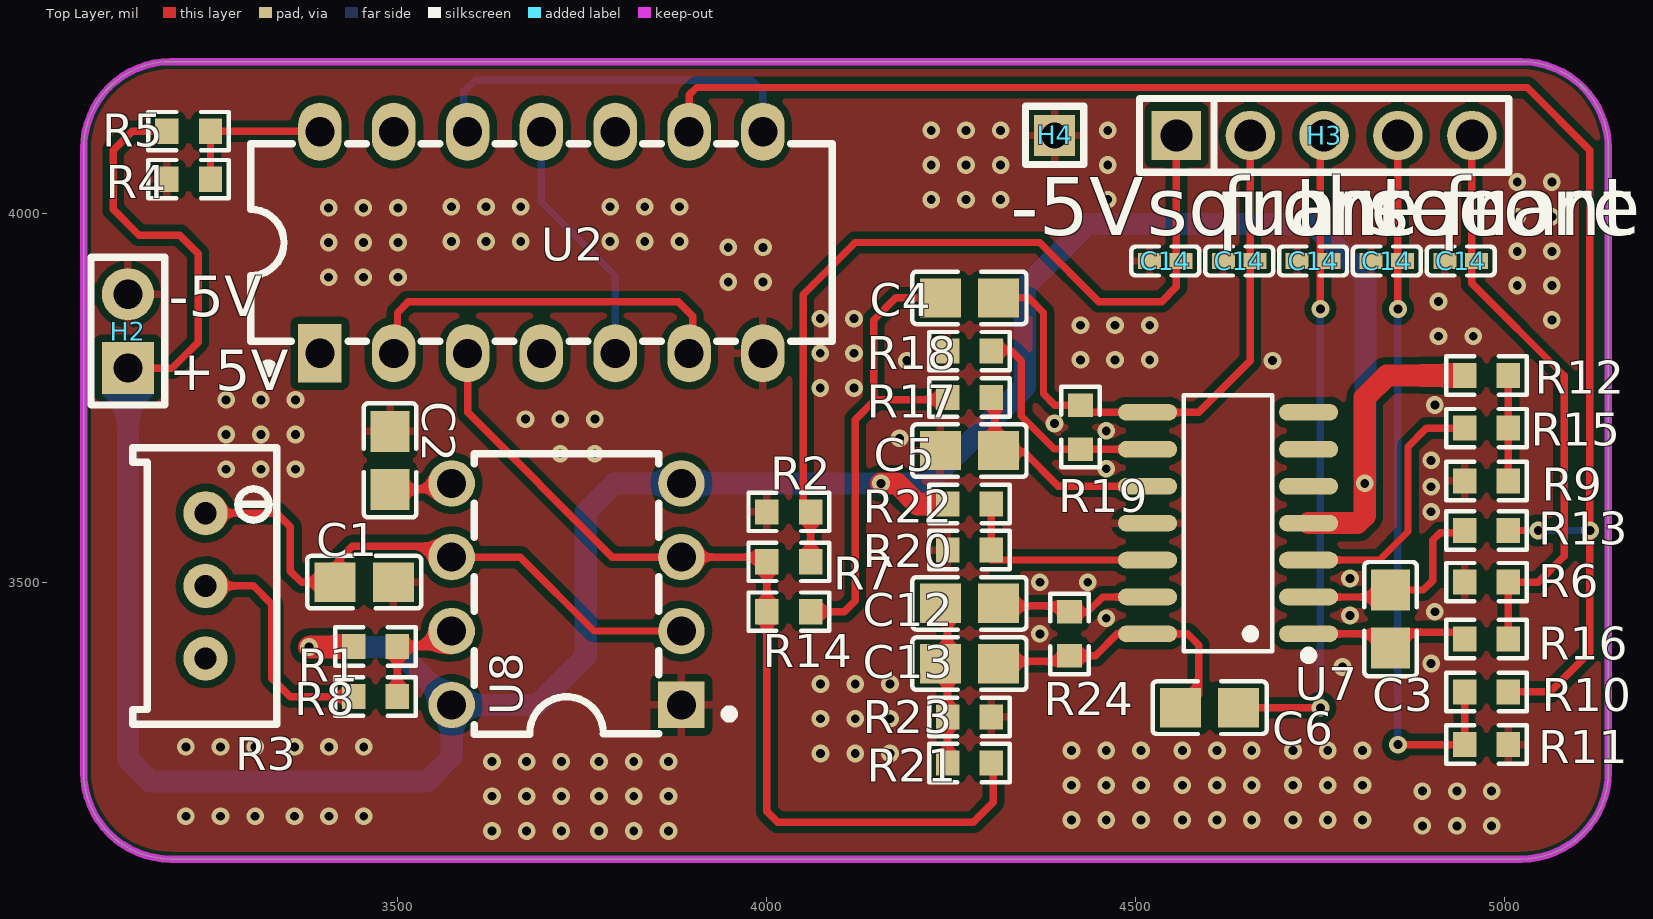
[diagram p0: Top Layer view]
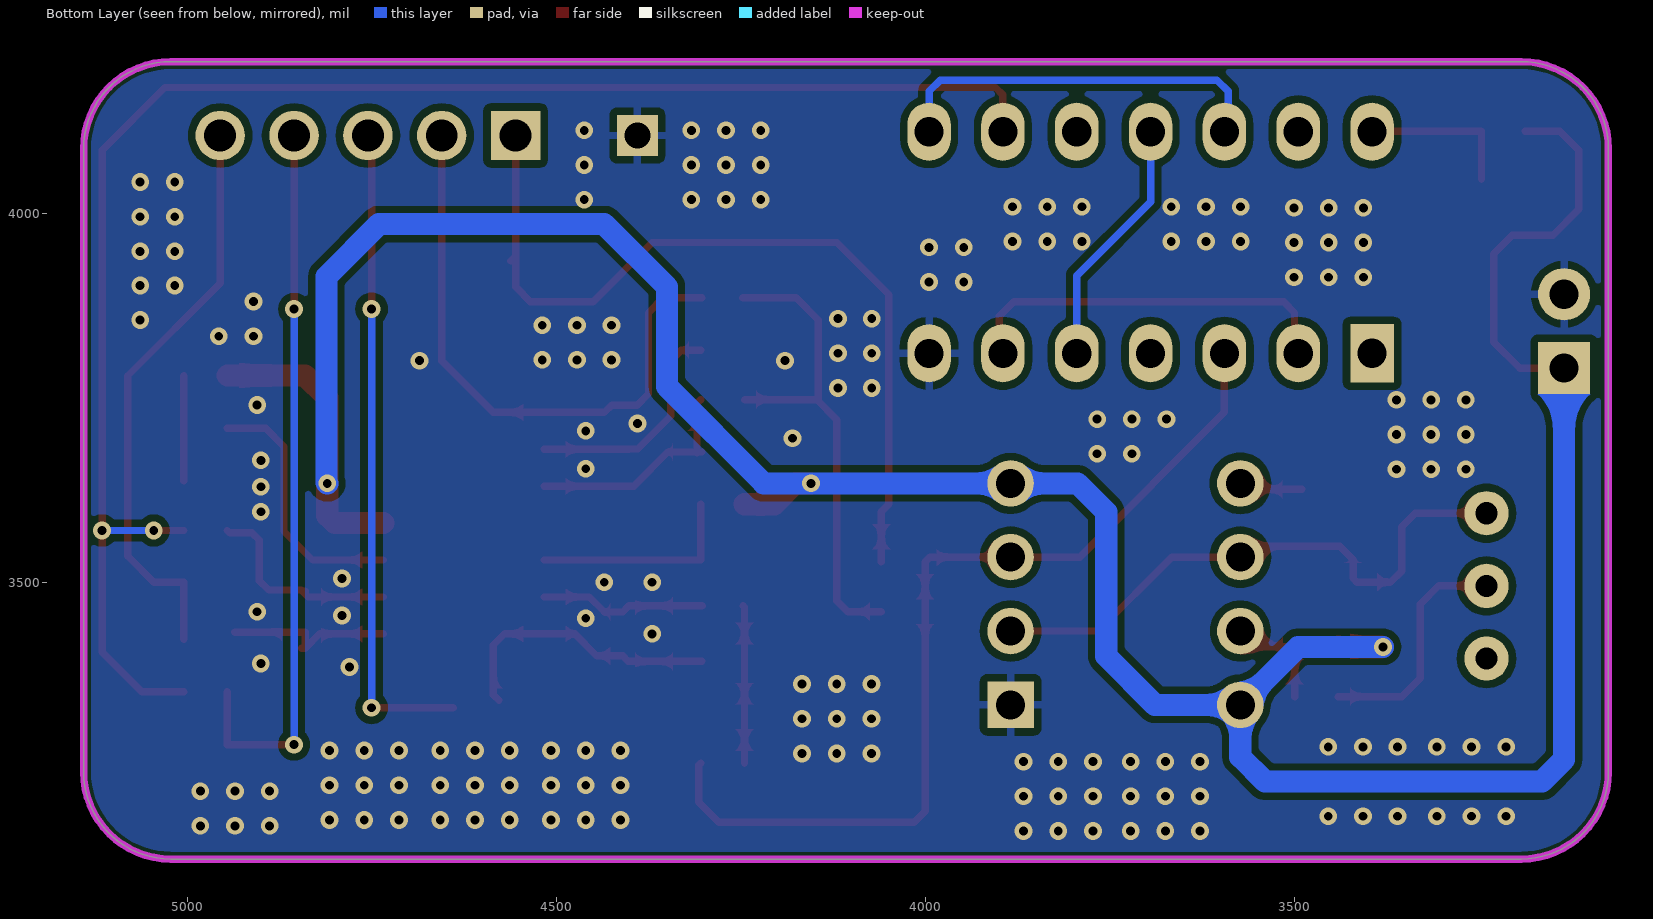
[diagram p1: Bottom Layer view, seen from below]
# Altium PCB MISC49933.pcbdoc
Units mil, origin at the board's own origin, x right, y up, seen from the top; angles counter-clockwise.
Board outline 2065 x 1080 mil, 2 copper layers (Top Layer, Bottom Layer), stack 62.206 mil thick; 43 components, 28 nets, 119 pads, 175 vias.

## Layer stack, top to bottom
Top Solder Mask Layer: solder mask 0.394, Dk 3.3
Top Layer: signal copper 1.379
Dielectric1: surface 59.449, FR4, Dk 4.5
Bottom Layer: signal copper 1.378
Bottom Solder Mask Layer: solder mask 0.394, Dk 3.3

## Board outline
3193.11,4205 ccw(c3193.11,4086.89) 3075,4086.89 3075,3243.11 ccw(c3193.11,3243.11) 3193.11,3125 5021.89,3125 ccw(c5021.89,3243.11) 5140,3243.11 5140,4086.89 ccw(c5021.89,4086.89) 5021.89,4205

## Design rules (kind name [scope] priority, off if disabled: settings)
BoardOutlineClearance copperThickness2oz_1 [All] p2 off: genericclearance=7.99 ignorepadtopadclearanceinfootprint=FALSE except(0: Arc-SplitContinuation Track-SplitContinuation SMDPad-SplitContinuation THPad-SplitContinuation Via-SplitContinuation Fill-SplitContinuation Region-SplitContinuation Poly-SplitContinuation Text-SplitContinuation Hole-SplitContinuation; 5.98: Arc-CutoutEdge Track-CutoutEdge SMDPad-CutoutEdge THPad-CutoutEdge Via-CutoutEdge Text-CutoutEdge; 6.9: Hole-OutlineEdge Hole-CutoutEdge; 10: Poly-OutlineEdge Poly-CutoutEdge; 11.81: Arc-OutlineEdge Track-OutlineEdge SMDPad-OutlineEdge THPad-OutlineEdge Via-OutlineEdge Fill-OutlineEdge Region-OutlineEdge Text-OutlineEdge Fill-CutoutEdge Region-CutoutEdge)
BoardOutlineClearance Plane_innerPlane_1 [All] p4 off: genericclearance=4.02 ignorepadtopadclearanceinfootprint=FALSE except(0: Arc-SplitContinuation Track-SplitContinuation SMDPad-SplitContinuation THPad-SplitContinuation Via-SplitContinuation Fill-SplitContinuation Region-SplitContinuation Poly-SplitContinuation Text-SplitContinuation Hole-SplitContinuation; 5.98: Arc-CutoutEdge Track-CutoutEdge SMDPad-CutoutEdge THPad-CutoutEdge Via-CutoutEdge Text-CutoutEdge; 6.9: Hole-OutlineEdge Hole-CutoutEdge; 10: Poly-OutlineEdge Poly-CutoutEdge; 11.81: Arc-OutlineEdge Track-OutlineEdge SMDPad-OutlineEdge THPad-OutlineEdge Via-OutlineEdge Fill-OutlineEdge Region-OutlineEdge Text-OutlineEdge Fill-CutoutEdge Region-CutoutEdge)
BoardOutlineClearance Copper_copperRegion_1 [All] p6 off: genericclearance=4.02 ignorepadtopadclearanceinfootprint=FALSE except(0: Arc-SplitContinuation Track-SplitContinuation SMDPad-SplitContinuation THPad-SplitContinuation Via-SplitContinuation Fill-SplitContinuation Region-SplitContinuation Poly-SplitContinuation Text-SplitContinuation Hole-SplitContinuation; 5.98: Arc-CutoutEdge Track-CutoutEdge SMDPad-CutoutEdge THPad-CutoutEdge Via-CutoutEdge Text-CutoutEdge; 6.9: Hole-OutlineEdge Hole-CutoutEdge; 10: Poly-OutlineEdge Poly-CutoutEdge; 11.81: Arc-OutlineEdge Track-OutlineEdge SMDPad-OutlineEdge THPad-OutlineEdge Via-OutlineEdge Fill-OutlineEdge Region-OutlineEdge Text-OutlineEdge Fill-CutoutEdge Region-CutoutEdge)
BoardOutlineClearance copperThickness1oz_1 [All] p8: genericclearance=4.02 ignorepadtopadclearanceinfootprint=FALSE except(0: Arc-SplitContinuation Track-SplitContinuation SMDPad-SplitContinuation THPad-SplitContinuation Via-SplitContinuation Fill-SplitContinuation Region-SplitContinuation Poly-SplitContinuation Text-SplitContinuation Hole-SplitContinuation; 5.98: Arc-CutoutEdge Track-CutoutEdge SMDPad-CutoutEdge THPad-CutoutEdge Via-CutoutEdge Text-CutoutEdge; 6.9: Hole-OutlineEdge Hole-CutoutEdge; 10: Poly-OutlineEdge Poly-CutoutEdge; 11.81: Arc-OutlineEdge Track-OutlineEdge SMDPad-OutlineEdge THPad-OutlineEdge Via-OutlineEdge Fill-OutlineEdge Region-OutlineEdge Text-OutlineEdge Fill-CutoutEdge Region-CutoutEdge)
Clearance copperThickness2oz [All] p1 off: gap=7.99 ignorepadtopadclearanceinfootprint=FALSE except(5.98: SMDPad-Track SMDPad-SMDPad THPad-Track SMDPad-THPad THPad-THPad Track-Via SMDPad-Via THPad-Via Via-Via Fill-SMDPad Region-SMDPad Fill-THPad Region-THPad Fill-Via Region-Via Fill-Fill Fill-Region Region-Region Arc-Track Arc-SMDPad Arc-THPad Arc-Via Fill-Arc Region-Arc Arc-Arc Text-Track SMDPad-Text Text-THPad Text-Via Fill-Text Region-Text Arc-Text Text-Text; 6.9: Hole-Track Hole-SMDPad Hole-THPad Hole-Via Fill-Hole Region-Hole Hole-Arc Hole-Text; 10: Poly-Track Poly-SMDPad Poly-THPad Poly-Via Poly-Fill Poly-Region Poly-Poly Poly-Arc Poly-Text Poly-Hole; 11.81: Fill-Track Region-Track)
Clearance Plane_innerPlane [All] p3 off: gap=4.02 ignorepadtopadclearanceinfootprint=FALSE except(5.98: SMDPad-Track SMDPad-SMDPad THPad-Track SMDPad-THPad THPad-THPad Track-Via SMDPad-Via THPad-Via Via-Via Fill-SMDPad Region-SMDPad Fill-THPad Region-THPad Fill-Via Region-Via Fill-Fill Fill-Region Region-Region Arc-Track Arc-SMDPad Arc-THPad Arc-Via Fill-Arc Region-Arc Arc-Arc Text-Track SMDPad-Text Text-THPad Text-Via Fill-Text Region-Text Arc-Text Text-Text; 6.9: Hole-Track Hole-SMDPad Hole-THPad Hole-Via Fill-Hole Region-Hole Hole-Arc Hole-Text; 10: Poly-Track Poly-SMDPad Poly-THPad Poly-Via Poly-Fill Poly-Region Poly-Poly Poly-Arc Poly-Text Poly-Hole; 11.81: Fill-Track Region-Track)
Clearance Copper_copperRegion [All] p5 off: gap=4.02 ignorepadtopadclearanceinfootprint=FALSE except(5.98: SMDPad-Track SMDPad-SMDPad THPad-Track SMDPad-THPad THPad-THPad Track-Via SMDPad-Via THPad-Via Via-Via Fill-SMDPad Region-SMDPad Fill-THPad Region-THPad Fill-Via Region-Via Fill-Fill Fill-Region Region-Region Arc-Track Arc-SMDPad Arc-THPad Arc-Via Fill-Arc Region-Arc Arc-Arc Text-Track SMDPad-Text Text-THPad Text-Via Fill-Text Region-Text Arc-Text Text-Text; 6.9: Hole-Track Hole-SMDPad Hole-THPad Hole-Via Fill-Hole Region-Hole Hole-Arc Hole-Text; 10: Poly-Track Poly-SMDPad Poly-THPad Poly-Via Poly-Fill Poly-Region Poly-Poly Poly-Arc Poly-Text Poly-Hole; 11.81: Fill-Track Region-Track)
Clearance copperThickness1oz [All] p7: gap=4.02 ignorepadtopadclearanceinfootprint=FALSE except(5.98: SMDPad-Track SMDPad-SMDPad THPad-Track SMDPad-THPad THPad-THPad Track-Via SMDPad-Via THPad-Via Via-Via Fill-SMDPad Region-SMDPad Fill-THPad Region-THPad Fill-Via Region-Via Fill-Fill Fill-Region Region-Region Arc-Track Arc-SMDPad Arc-THPad Arc-Via Fill-Arc Region-Arc Arc-Arc Text-Track SMDPad-Text Text-THPad Text-Via Fill-Text Region-Text Arc-Text Text-Text; 6.9: Hole-Track Hole-SMDPad Hole-THPad Hole-Via Fill-Hole Region-Hole Hole-Arc Hole-Text; 10: Poly-Track Poly-SMDPad Poly-THPad Poly-Via Poly-Fill Poly-Region Poly-Poly Poly-Arc Poly-Text Poly-Hole; 11.81: Fill-Track Region-Track)
DiffPairsRouting differentialPair [All] p1: maxlimit=6 minlimit=6 mostfreqgap=6 toplayer_minwidth=5 toplayer_prefwidth=10 toplayer_maxwidth=100 toplayer_mingap=6 toplayer_prefgap=6 toplayer_maxgap=6 bottomlayer_minwidth=5 bottomlayer_prefwidth=10 bottomlayer_maxwidth=100 bottomlayer_mingap=6 bottomlayer_prefgap=6 bottomlayer_maxgap=6 maxuncoupledlength=10
HoleToHoleClearance otherClearance [All] p1: gap=11.81 allowstackedmicrovias=TRUE
Length netLength [All] p1: minlimit=0 maxlimit=0
PasteMaskExpansion pasteMaskExpansion [All] p1: expansion=0
PlaneConnect innerPlane [All] p1: planeconnectstyle=Relief reliefexpansion=20 reliefentries=4 reliefconductorwidth=10 reliefairgap=10
PolygonConnect copperRegion [All] p1: connectstyle=Relief reliefconductorwidth=10 reliefentries=4 polygonreliefangle="90 Angle" airgapwidth=10 via.connectstyle=Relief via.reliefconductorwidth=10 via.reliefentries=4 via.polygonreliefangle="90 Angle" via.airgapwidth=10
RoutingVias viaSize [All] p1: holewidth=12.01 width=24.02 viastyle="Through Hole" minholewidth=11.81 minwidth=19.68 maxholewidth=248.03 maxwidth=393.7
SolderMaskExpansion solderMaskExpansion [IsVia] p1: expansion=-1000 istentingtop=TRUE
SolderMaskExpansion solderMaskExpansion [All] p2: expansion=2 istentingtop=FALSE
Width copperThickness2oz_2 [All] p1 off: maxlimit=100 minlimit=8 preferedwidth=10
Width copperThickness1oz_2 [All] p2: maxlimit=100 minlimit=5 preferedwidth=10

## Components (designator, comment, footprint, x,y, rotation, side; value= is the part's Value field where it differs from the comment)
C1 "1nF" C0805 3455,3500 r180 top
C2 "0.01uF" C0805 3490,3665 r270 top
C3 "10nF" C0805 4845,3450 r90 top
C4 "1nF" C0805 4274.69,3885 r0 top
C5 "1nF" C0805 4274.69,3678.19 r0 top
C6 "1nF" C0805 4600,3330 r180 top
C12 "0.11nF" C0805 4274.69,3471.38 r180 top
C13 "0.1nF" C0805 4274.69,3389.68 r180 top
C14 "220nF" C0402 4540,3935 r0 top
C14 "220nF" C0402 4640,3935 r0 top
C14 "220nF" C0402 4740,3935 r0 top
C14 "220nF" C0402 4840,3935 r0 top
C14 "220nF" C0402 4940,3935 r0 top
H2 "" HDR-TH_2P-P2.54-V-M-1 3135,3840 r90 top
H3 "" HDR-TH_5P-P2.54-V-M 4755,4105 r0 top
H4 "" HDR-TH_1P-V-M_XKB_X4611WV-01I-C28D40 4390,4105 r0 top
R1 "510" R0603 3470.3,3412.92 r180 top
R2 "60" R0603 4030,3595.31 r0 top
R3 "24K" R_3296 3245,3495 r270 top
R4 "1K" R0603 3217.13,4045.75 r0 top
R5 "1K" R0603 3217.13,4110.75 r180 top
R6 "200" R0603 4975,3500 r0 top
R7 "540" R0603 4030,3527.65 r180 top
R8 "12k" R0603 3470.3,3345 r0 top
R9 "100" R0603 4975,3637.14 r180 top
R10 "480" R0603 4975,3351.43 r0 top
R11 "120" R0603 4975,3280 r180 top
R12 "300" R0603 4975,3780 r0 top
R13 "1.8K" R0603 4975,3570 r0 top
R14 "10k" R0603 4030,3460 r180 top
R15 "1K" R0603 4975,3708.57 r0 top
R16 "400" R0603 4975,3422.86 r180 top
R17 "16.5k" R0603 4274.69,3750.32 r180 top
R18 "3.6k" R0603 4274.69,3812.87 r180 top
R19 "720" R0603 4425,3710 r270 top
R20 "1.35k" R0603 4274.69,3543.5 r180 top
R21 "41k" R0603 4274.69,3255 r0 top
R22 "1k" R0603 4274.69,3606.06 r0 top
R23 "50" R0603 4274.69,3317.56 r0 top
R24 "90k" R0603 4410,3430 r270 top
U2 "SN74LS74AN" PDIP-14_L19.5-W6.7-P2.54-LS7.9-BL 3695,3960 r0 top
U7 "LM324AD" SOIC-14_L8.7-W3.9-P1.27-LS6.0-BL 4625,3580 r90 top
U8 "NE555PE4" PDIP-8_L9.6-W6.4-P2.54-LS7.9-BL-1 3728.98,3483.87 r90 top

## Footprints (in the part's own frame and the unit in brackets; to place one, negate y for a bottom-side part, rotate by r counter-clockwise, add the part's x,y. Pads: shape width x height; smd on the part's side, far side on the other; paste and mask are expansions set on the pad)
C0402 [mm]
  rect 0.79x0.54 smd paste-100 mask+0.051: 1(-0.545,0) 2(0.545,0)
  silkscreen extent -1.17,-0.5 1.17,0.5
C0805 [mm]
  rect 1.41x1.35 smd paste-100 mask+0.051: 1(-1,0) 2(1,0)
  silkscreen extent -1.96,-0.9 1.96,0.9
HDR-TH_1P-V-M_XKB_X4611WV-01I-C28D40 [mm]
  rect 1.4x1.4 hole 0.9: 1(0,0)
  silkscreen extent -1,-1 1,1
HDR-TH_2P-P2.54-V-M-1 [mm]
  rect 1.8x1.8 hole 1: 1(-1.27,0)
  round 1.8 hole 1: 2(1.27,0)
  silkscreen extent -2.54,-1.27 2.54,1.27
HDR-TH_5P-P2.54-V-M [mm]
  rect 1.7x1.7 hole 1.1: 1(-5.08,0)
  round 1.7 hole 1.1: 2(-2.54,0) 3(0,0) 4(2.54,0) 5(5.08,0)
  silkscreen extent -6.35,-1.27 6.35,1.27
PDIP-8_L9.6-W6.4-P2.54-LS7.9-BL-1 [mil]
  rect 63x63 hole 39.37: 1(-150,-155.51)
  round 63 hole 39.37: 2(-50,-155.51) 3(50,-155.51) 4(150,-155.51) 5(150,155.52) 6(50,155.52) 7(-50,155.52) 8(-150,155.52)
  silkscreen extent -190,-226 190,125
PDIP-14_L19.5-W6.7-P2.54-LS7.9-BL [mm]
  rect 1.5x2 hole 1: 1(-7.62,-3.81)
  oval 1.5x2 hole 1: 2(-5.08,-3.81) 3(-2.54,-3.81) 4(0,-3.81) 5(2.54,-3.81) 6(5.08,-3.81) 7(7.62,-3.81)
  oval 1.5x2 hole 1 copper offset 0,0: 8(7.62,3.81) 9(5.08,3.81) 10(2.54,3.81) 11(0,3.81) 12(-2.54,3.81) 13(-5.08,3.81) 14(-7.62,3.81)
  silkscreen extent -10,-4.47 10,3.4
R0603 [mil]
  rect 31.75x34.02 smd paste-3937.01 mask+2: 1(-29.66,0) 2(29.66,0)
  silkscreen extent -55,-26 55,26
R_3296 [mil]
  round 60 hole 30 paste+0 mask+2: 1(-98.4,-5) 2(0,-5) 3(98.4,-5)
  silkscreen extent -187,-103 187,92
SOIC-14_L8.7-W3.9-P1.27-LS6.0-BL [mil]
  oval 22.6x80.24 smd: 1(-150,-109.02) 2(-100,-109.02) 3(-50,-109.02) 4(0,-109.02) 5(50,-109.02) 6(100,-109.02) 7(150,-109.02) 8(150,109.02) 9(100,109.02) 10(50,109.02) 11(0,109.02) 12(-50,109.02) 13(-100,109.02) 14(-150,109.02)
  silkscreen extent -185,-115 173,60

## Via types
v1: diameter 24.02, hole 12, Top Layer to Bottom Layer, 173 vias
v2: diameter 24, hole 12, Top Layer to Bottom Layer, 2 vias

## Nets (pads, with @x,y where several pads share a name; then routed paths per layer and width w, separated by ;. In a path a pad name is that pad's centre, name@x,y a point inside that pad or via, vN(x,y) a via of type N, cw(c..) or ccw(c..) an arc to the next point about the centre after c; other vN are vias at no path point)
$1N553: R1.1 R8.2 U8.7 | length 150.1
  Top Layer w10: R8.2 R1.1 3552.53,3412.92 U8.7
$1N739: C1.2 R3.1 U8.2 U8.6 | length 801.2
  Top Layer w10: R3.1 3336.6,3593.4 3355,3575 3355,3515 3370,3500 C1.2 3420.63,3505 3420.63,3530.63 3438.87,3548.87 3558.47,3548.87 U8.6 3666.13,3533.87 3766.13,3433.87 U8.2
$1N829: C2.2 U8.5 | length 91
  Top Layer w10: C2.2 3555.24,3625.63 3560.24,3620.63 U8.5
$1N871: R7.2 R14.2 R21.2 U2.3 U8.3 | length 1285.2
  Top Layer w10: U2.3 3595,3730 3791.13,3533.87 U8.3 3994.13,3533.87 R7.2 R14.2 4000.34,3189.66 4015,3175 4280,3175 4307.07,3202.07 4307.07,3252.28 R21.2
$1N1305: R4.2 R5.1 U2.14 | length 213.5
  Top Layer w10: R4.2 R5.1 3394.25,4110.75 U2.14
$1N1323: U2.8 U2.12 | length 529.5
  Bottom Layer w10: U2.12 3590,4115 3590,4165 3605,4180 3980,4180 3995,4165 U2.8
$1N1329: U2.5 U2.11 | length 341.4
  Bottom Layer w10: U2.11 3695,4015 3795,3915 U2.5
$1N1412: U2.2 U2.6 | length 523.5
  Top Layer w10: U2.2 3500,3815 3500,3865 3514.79,3879.79 3880.21,3879.79 3900,3860 3900,3815 U2.6
$1N2821: C5.2 R17.1 U7.10 | length 308.9
  Top Layer w10: C5.2@4302.56,3676.32 C5.2@4308.05,3676.32 ; R17.1@4304.35,3747.33 4309.37,3742.32 C5.2@4309.37,3676.32 ; U7.10 4395,3630 4348.68,3676.32 C5.2@4309.37,3676.32 ; C5.2@4308.05,3676.32 4309.37,3675 C5.2@4309.37,3676.32 ; C5.2@4308.05,3676.32 C5.2@4309.37,3676.32
$1N2825: R18.1 R19.2 U7.9 | length 335.5
  Top Layer w10: R18.1@4304.35,3814.19 4330.81,3814.19 4345,3800 4345,3725 4389.66,3680.34 4400.67,3680.34 ; R19.2 4400.67,3680.34 ; U7.9 4401.01,3680 4400.67,3680.34
$1N3061: C4.1 R14.1 R17.2 | length 672.8
  Top Layer w10: R14.1 4105,3460 4120,3475 4120,3720 4147.33,3747.33 ; R17.2@4245.03,3747.33 4147.33,3747.33 ; C4.1@4247.44,3885 4175,3885 4145,3855 4145,3747.33 4147.33,3747.33
$1N3703: C12.1 R24.1 U7.13 | length 225.8
  Top Layer w10: C12.1@4301.95,3467.84 4401.82,3467.84 R24.1 4434.66,3459.66 4455,3480 U7.13
$1N3731: C12.2 C13.2 R21.1 R23.1 | length 213.6
  Top Layer w10: R21.1 4245.03,3321.86 4245.03,3466.05 C12.2@4246.83,3467.84
$1N3807: C6.2 C13.1 R24.2 U7.14 | length 382.2
  Top Layer w10: C13.1@4302.56,3392.67 4402.33,3392.67 R24.2 4445.34,3400.34 4475,3430 U7.14 4570,3430 4585,3415 4585,3347.56 C6.2@4577.44,3340
$1N4038: R20.1 R22.2 U7.12 | length 287.1
  Top Layer w10: R22.2@4304.35,3605.51 4304.35,3530 U7.12
$1N4114: R3.2 R8.1 | length 321.4
  Top Layer w10: R3.2 3305,3495 3330,3470 3330,3370 3355,3345 R8.1
$1N7012: C3.1 R16.2 U7.1 | length 236.6
  Top Layer w10: U7.1 4820.63,3430 C3.1@4840,3410.63 ; C3.1 C3.1@4840,3410.63 ; R16.2@4935.76,3432.44 4840,3432.44 C3.1@4840,3410.63
$1N7150: C3.2 R13.1 U7.2 | length 284
  Top Layer w10: U7.2 4835.63,3480 C3.2@4843.19,3487.56 ; C3.2@4840,3487.56 C3.2@4843.19,3487.56 ; R13.1 4942.41,3567.07 4912.07,3567.07 4902.07,3557.07 4902.07,3502.07 4889.37,3489.37 C3.2 C3.2@4843.19,3487.56
$1N7244: R15.1 U7.3 | length 352.7
  Top Layer w10: U7.3 4830,3530 4868.57,3568.57 4868.57,3683.57 4893.57,3708.57 R15.1
$1N7250: R10.2 R13.2 U2.9 | length 2232.2
  Top Layer w10: U2.9 3895,4160 3905,4170 5030,4170 5115,4085 v1(5115,3570) 5115,3405 5061.43,3351.43 R10.2 ; R13.2 v1(5045,3570)
  Bottom Layer w10: v1(5045,3570) v1(5115,3570)
$1N7309: R9.1 R12.2 R15.2 | length 142.9
  Top Layer w10: R9.1 R15.2 R12.2
A1: C14.2@4561.46,3935 H3.1 R2.2 R7.1 | length 1156.2
  Top Layer w10: R7.1 R2.2 4049.66,3605.31 4049.66,3889.66 4120,3960 4370,3960 4450,3880 4535,3880 4555,3900 C14.2@4555,3941.46 ; H3.1 C14.2@4555,3941.46 ; C14.2@4561.46,3935 C14.2@4555,3941.46
A2: C6.1 C14.2@4761.46,3935 H3.3 | length 887.7
  Top Layer w10: C6.1 v1(4750,3330) ; v1(4750,3870) 4750,4100 H3.3
  Bottom Layer w10: v1(4750,3330) v1(4750,3870)
B: C14.2@4861.46,3935 H3.4 R10.1 R11.2 | length 986.8
  Top Layer w10: v1(4855,3280) R11.2 R10.1 ; v1(4855,3870) H3.4
  Bottom Layer w10: v1(4855,3280) v1(4855,3870)
C: C14.2@4961.46,3935 H3.5 R6.2 R16.1 | length 788.8
  Top Layer w10: H3.5 4955,3905 5080,3780 5080,3535 5045,3500 R6.2 R16.1
D: C4.2 C14.2@4661.46,3935 H3.2 R19.1 U7.8 | length 815.1
  Top Layer w10: C4.2@4302.56,3885 4355,3885 4375,3865 4375,3755 4390.34,3739.66 R19.1 4434.66,3730 U7.8 4585,3730 4655,3800 H3.2
GND: C1.1 C2.1 C5.1 C14.1 H2.2 H4.1 R2.1 R4.1 R6.1 R9.2 R11.1 R18.2 R20.2 R23.2 U2.7 U7.11 U8.1
  other v1: 3628.05,3163.05 3675,3163.05 3721.95,3163.05 3773.05,3163.05 3820,3163.05 3866.95,3163.05 4888.05,3170 4935,3170 4981.95,3170 4413.05,3178.05 4460,3178.05 4506.95,3178.05 4563.05,3178.05 4610,3178.05 4656.95,3178.05 4713.05,3178.05 4760,3178.05 4806.95,3178.05 3213.4,3183.05 3260.35,3183.05 3307.31,3183.05 3360.5,3183.05 3407.45,3183.05 3454.41,3183.05 3628.05,3210 3675,3210 3721.95,3210 3773.05,3210 3820,3210 3866.95,3210 4888.05,3216.95 4935,3216.95 4981.95,3216.95 4413.05,3225 4460,3225 4506.95,3225 4563.05,3225 4610,3225 4656.95,3225 4713.05,3225 4760,3225 4806.95,3225 3628.05,3256.95 3675,3256.95 3721.95,3256.95 3773.05,3256.95 3820,3256.95 3866.95,3256.95 4073.05,3268.05 4120,3268.05 4166.95,3268.05 4413.05,3271.95 4460,3271.95 4506.95,3271.95 4563.05,3271.95 4610,3271.95 4656.95,3271.95 4713.05,3271.95 4760,3271.95 4806.95,3271.95 3213.4,3276.95 3260.35,3276.95 3307.31,3276.95 3360.5,3276.95 3407.45,3276.95 3454.41,3276.95 4073.05,3315 4120,3315 4166.95,3315 4073.05,3361.95 4120,3361.95 4166.95,3361.95 4780,3385 4900,3390 4370,3430 4460,3451.08 4790,3455 4905,3460 4370,3500 4435,3500 4790,3505 4900,3595.43 4900,3629.25 3268.05,3653.05 3315,3653.05 3361.95,3653.05 4460,3653.66 4900,3665 3720.37,3673.87 3767.32,3673.87 4180,3695 3268.05,3700 3315,3700 3361.95,3700 4460,3705 4390,3715 3673.42,3720.82 3720.37,3720.82 3767.32,3720.82 4905,3740 3268.05,3746.95 3315,3746.95 3361.95,3746.95 4072.65,3763.05 4118.48,3763.05 4190,3800 4685,3800 4425,3801.09 4471.95,3801.09 4518.91,3801.09 4072.65,3810 4118.48,3810 4910,3833.05 4956.95,3833.05 4425,3848.05 4471.95,3848.05 4518.91,3848.05 5063.48,3855 4072.65,3856.95 4118.48,3856.95 4910,3880 5016.52,3901.95 5063.48,3901.95 3948.05,3906.52 3995,3906.52 3406.83,3913.05 3453.79,3913.05 3500.74,3913.05 5016.52,3948.05 5063.48,3948.05 3948.05,3953.48 3995,3953.48 3406.83,3960 3453.79,3960 3500.74,3960 3573.05,3961.52 3620,3961.52 3666.95,3961.52 3788.05,3961.52 3835,3961.52 3881.95,3961.52 5016.52,3995 5063.48,3995 3406.83,4006.95 3453.79,4006.95 3500.74,4006.95 3573.05,4008.48 3620,4008.48 3666.95,4008.48 3788.05,4008.48 3835,4008.48 3881.95,4008.48 4223.05,4018.05 4270,4018.05 4316.95,4018.05 4461.95,4018.05 5016.52,4041.95 5063.48,4041.95 4223.05,4065 4270,4065 4316.95,4065 4461.95,4065 4223.05,4111.95 4270,4111.95 4316.95,4111.95 4461.95,4111.95
VCC: H2.1 R1.2 R5.2 R12.1 R22.1 U7.4 U8.4 U8.8 | length 4384.5
  Top Layer w10: H2.1 3195,3790 3230,3825 3230,3945 3205,3970 3150,3970 3115,4005 3115,4085 3140.75,4110.75 R5.2
  Top Layer w30: v1(3380.2,3412.3) 3440.02,3412.3 R1.2 ; v2(4155,3633.87) 4176.13,3633.87 4204.49,3605.51 R22.1@4245.03,3605.51 ; U7.4 4800,3580 4810,3590 v2(4810,3633.87) 4810,3750 4840,3780 R12.1
  Bottom Layer w30: H2.1 3135,3260 3165,3230 3540,3230 3573.47,3263.47 U8.8 ; v1(3380.2,3412.3) 3495.04,3412.3 U8.8 ; v2(4810,3633.87) 4811.21,3635.08 4811.21,3913.79 4739.94,3985.06 4435.06,3985.06 4350,3900 4350,3765 4218.87,3633.87 v2(4155,3633.87) U8.4 3793.87,3633.87 3755,3595 3755,3400 3688.87,3333.87 U8.8
pads on no net: R3.3 U2.1 U2.4 U2.10 U2.13 U7.5 U7.6 U7.7

## Polygon pours and split planes (outlines as drawn)
GND on Bottom Layer (solid, remove dead copper, pour order 2): 3040,4360 3040,3000 5185,3000 5185,4360
GND on Top Layer (solid, remove dead copper, pour order 0): 3000,4275 3000,3055 5245,3055 5245,4275

## Keep-outs
Board Outline Layer:
  the board outline again, w10

## Other copper
Top Layer:
  region net VCC: 3380.2,3397.3 3380.2,3427.3 3395.09,3427.59 3409.95,3428.47 3424.77,3429.93 3424.77,3395.91 3402.5,3396.95 3380.2,3397.3
  region net $1N553: 3530.84,3417.92 3530.84,3407.92 3527.38,3407.6 3524.04,3406.65 3520.94,3405.09 3518.17,3402.99 3515.84,3400.42 3515.84,3425.42 3518.17,3422.85 3520.94,3420.75 3524.04,3419.2 3527.38,3418.24 3530.84,3417.92
  region net $1N553: 3504.97,3380.91 3494.97,3380.91 3494.64,3384.37 3493.69,3387.71 3492.14,3390.81 3490.04,3393.58 3487.47,3395.91 3512.47,3395.91 3509.89,3393.58 3507.79,3390.81 3506.24,3387.71 3505.29,3384.37 3504.97,3380.91
  region net A1: 4064.66,3563.3 4054.66,3563.3 4054.34,3566.76 4053.38,3570.1 4051.83,3573.2 4049.73,3575.97 4047.16,3578.3 4072.16,3578.3 4069.59,3575.97 4067.49,3573.2 4065.94,3570.1 4064.98,3566.76 4064.66,3563.3
  region net $1N871: 4005.34,3495.65 3995.34,3495.65 3995.02,3499.1 3994.06,3502.44 3992.51,3505.55 3990.41,3508.31 3987.84,3510.65 4012.84,3510.65 4010.27,3508.31 4008.17,3505.55 4006.62,3502.44 4005.66,3499.1 4005.34,3495.65
  region net $1N871: 3969.46,3528.87 3969.46,3538.87 3973.55,3539.24 3977.51,3540.37 3981.18,3542.19 3984.46,3544.66 3984.46,3521.37 3982.13,3523.94 3979.37,3526.04 3976.26,3527.59 3972.92,3528.54 3969.46,3528.87
  region net A1: 4054.66,3559.66 4064.66,3559.66 4064.98,3556.2 4065.94,3552.87 4067.49,3549.76 4069.59,3546.99 4072.16,3544.66 4047.16,3544.66 4049.73,3546.99 4051.83,3549.76 4053.38,3552.87 4054.34,3556.2 4054.66,3559.66
  region net $1N553: 3494.97,3377.01 3504.97,3377.01 3505.29,3373.55 3506.24,3370.21 3507.79,3367.11 3509.89,3364.34 3512.47,3362.01 3487.47,3362.01 3490.04,3364.34 3492.14,3367.11 3493.69,3370.21 3494.64,3373.55
  region net $1N4114: 3409.77,3340 3409.77,3350 3413.23,3350.32 3416.57,3351.28 3419.67,3352.83 3422.44,3354.93 3424.77,3357.5 3424.77,3332.5 3422.44,3335.07 3419.67,3337.17 3416.57,3338.72 3413.23,3339.68 3409.77,3340
  region net VCC: 4884.46,3765 4884.46,3795 4899.48,3795.22 4914.49,3795.89 4929.46,3797.01 4929.46,3762.99 4914.49,3764.11 4899.48,3764.78 4884.46,3765
  region net $1N871: 3995.34,3492.01 4005.34,3492.01 4005.66,3488.55 4006.62,3485.21 4008.17,3482.11 4010.27,3479.34 4012.84,3477.01 3987.84,3477.01 3990.41,3479.34 3992.51,3482.11 3994.06,3485.21 3995.02,3488.55
  region net $1N871: 4005.34,3427.99 3995.34,3427.99 3995.02,3431.45 3994.06,3434.79 3992.51,3437.89 3990.41,3440.66 3987.84,3442.99 4012.84,3442.99 4010.27,3440.66 4008.17,3437.89 4006.62,3434.79 4005.66,3431.45
  region net $1N3061: 4090.54,3465 4090.54,3455 4087.08,3454.68 4083.74,3453.72 4080.63,3452.17 4077.87,3450.07 4075.54,3447.5 4075.54,3472.5 4077.87,3469.93 4080.63,3467.83 4083.74,3466.28 4087.08,3465.32 4090.54,3465
  region net $1N3061: 4214.16,3742.33 4214.16,3752.33 4217.62,3752.66 4220.96,3753.61 4224.06,3755.16 4226.83,3757.26 4229.16,3759.83 4229.16,3734.83 4226.83,3737.41 4224.06,3739.51 4220.96,3741.06 4217.62,3742.01 4214.16,3742.33
  region net $1N2821: 4314.37,3718.31 4304.37,3718.31 4304.05,3721.76 4303.09,3725.1 4301.54,3728.21 4299.44,3730.98 4296.87,3733.31 4320.23,3733.31 4317.73,3730.04 4315.89,3726.36 4314.75,3722.4 4314.37,3718.31
  region net $1N2825: 4330.81,3819.19 4330.81,3809.19 4328.07,3808.85 4325.5,3807.86 4323.25,3806.26 4321.46,3804.16 4320.23,3801.69 4320.23,3826.69 4321.46,3824.22 4323.25,3822.13 4325.5,3820.53 4328.07,3819.53 4330.81,3819.19
  region net $1N3731: 4240.03,3287.01 4250.03,3287.01 4250.36,3283.55 4251.31,3280.21 4252.86,3277.11 4254.96,3274.34 4257.53,3272.01 4232.53,3272.01 4235.11,3274.34 4237.21,3277.11 4238.76,3280.21 4239.71,3283.55
  region net VCC: 4204.49,3590.51 4204.49,3620.51 4212.77,3620.79 4221,3621.65 4229.16,3623.07 4229.16,3589.05 4216.85,3590.15 4204.49,3590.51
  region net $1N3731: 4250.03,3285.55 4240.03,3285.55 4239.71,3289.01 4238.76,3292.35 4237.21,3295.45 4235.11,3298.22 4232.53,3300.55 4257.53,3300.55 4254.96,3298.22 4252.86,3295.45 4251.31,3292.35 4250.36,3289.01 4250.03,3285.55
  region net $1N3731: 4240.03,3349.57 4250.03,3349.57 4250.36,3346.11 4251.31,3342.77 4252.86,3339.66 4254.96,3336.9 4257.53,3334.57 4232.53,3334.57 4235.11,3336.9 4237.21,3339.66 4238.76,3342.77 4239.71,3346.11 4240.03,3349.57
  region net $1N3807: 4377.99,3387.67 4377.99,3397.67 4381.45,3397.99 4384.79,3398.94 4387.89,3400.49 4390.66,3402.59 4392.99,3405.17 4392.99,3384.46 4388.16,3386.23 4383.13,3387.31 4377.99,3387.67
  region net $1N3807: 4442.01,3405.34 4442.01,3395.34 4438.55,3395.02 4435.21,3394.06 4432.11,3392.51 4429.34,3390.41 4427.01,3387.84 4427.01,3412.84 4429.34,3410.27 4432.11,3408.17 4435.21,3406.62 4438.55,3405.66 4442.01,3405.34
  region net $1N3703: 4434.66,3464.66 4434.66,3454.66 4432.32,3454.29 4430.21,3453.23 4428.52,3451.58 4427.42,3449.49 4427.01,3447.16 4427.01,3472.16 4427.42,3469.83 4428.52,3467.74 4430.21,3466.09 4432.32,3465.03 4434.66,3464.66
  region net $1N3703: 4377.99,3462.84 4377.99,3472.84 4383.09,3473.15 4388.11,3474.05 4392.99,3475.54 4392.99,3455.34 4390.66,3457.92 4387.89,3460.02 4384.79,3461.57 4381.45,3462.52 4377.99,3462.84
  region net $1N7012: 4777.84,3435 4777.84,3425 4775.08,3424.73 4772.47,3424.02 4770.06,3423.01 4767.9,3421.85 4764.55,3419.69 4763.47,3418.97 4762.84,3418.7 4762.84,3441.3 4763.47,3441.03 4764.55,3440.31 4767.9,3438.15 4770.06,3436.99 4772.47,3435.98 4775.08,3435.27
  region net $1N7150: 4777.84,3485 4777.84,3475 4775.08,3474.73 4772.47,3474.02 4770.06,3473.01 4767.9,3471.85 4764.55,3469.69 4763.47,3468.97 4762.84,3468.7 4762.84,3491.3 4763.47,3491.03 4764.55,3490.31 4767.9,3488.15 4770.06,3486.99 4772.47,3485.98 4775.08,3485.27
  region net $1N7244: 4777.84,3535 4777.84,3525 4775.08,3524.73 4772.47,3524.02 4770.06,3523.01 4767.9,3521.85 4764.55,3519.69 4763.47,3518.97 4762.84,3518.7 4762.84,3541.3 4763.47,3541.03 4764.55,3540.31 4767.9,3538.15 4770.06,3536.99 4772.47,3535.98 4775.08,3535.27
  region net $1N3807: 4475,3425 4475,3435 4477.23,3435.27 4479.33,3435.98 4481.26,3436.99 4482.99,3438.15 4485.7,3440.31 4486.6,3441.03 4487.16,3441.3 4487.16,3418.7 4486.6,3418.97 4485.7,3419.69 4482.99,3421.85 4481.26,3423.01 4479.33,3424.02 4477.23,3424.73
  region net $1N3807: 4559.8,3435 4559.8,3425 4557.04,3424.73 4554.43,3424.02 4552.02,3423.01 4549.86,3421.85 4546.51,3419.69 4545.43,3418.97 4544.8,3418.7 4544.8,3441.3 4545.43,3441.03 4546.51,3440.31 4549.86,3438.15 4552.02,3436.99 4554.43,3435.98 4557.04,3435.27
  region net $1N3703: 4472.16,3475 4472.16,3485 4474.92,3485.27 4477.53,3485.98 4479.94,3486.99 4482.1,3488.15 4485.45,3490.31 4486.54,3491.03 4487.16,3491.3 4487.16,3468.7 4486.54,3468.97 4485.45,3469.69 4482.1,3471.85 4479.94,3473.01 4477.53,3474.02 4474.92,3474.73
  region net $1N2821: 4472.16,3625 4472.16,3635 4474.92,3635.27 4477.53,3635.98 4479.94,3636.99 4482.1,3638.15 4485.45,3640.31 4486.54,3641.03 4487.16,3641.3 4487.16,3618.7 4486.54,3618.97 4485.45,3619.69 4482.1,3621.85 4479.94,3623.01 4477.53,3624.02 4474.92,3624.73
  region net $1N2825: 4472.16,3675 4472.16,3685 4474.92,3685.27 4477.53,3685.98 4479.94,3686.99 4482.1,3688.15 4485.45,3690.31 4486.54,3691.03 4487.16,3691.3 4487.16,3668.7 4486.54,3668.97 4485.45,3669.69 4482.1,3671.85 4479.94,3673.01 4477.53,3674.02 4474.92,3674.73
  region net D: 4559.8,3735 4559.8,3725 4557.04,3724.73 4554.43,3724.02 4552.02,3723.01 4549.86,3721.85 4546.51,3719.69 4545.43,3718.97 4544.8,3718.7 4544.8,3741.3 4545.43,3741.03 4546.51,3740.31 4549.86,3738.15 4552.02,3736.99 4554.43,3735.98 4557.04,3735.27
  region net $1N4114: 3281,3500 3281,3490 3278.73,3489.9 3276.76,3489.61 3275.06,3489.14 3273.59,3488.51 3272.31,3487.72 3271.19,3486.8 3269.26,3484.57 3265.54,3479.01 3263.15,3475.88 3261.69,3474.26 3260,3472.64 3260,3517.36 3261.69,3515.74 3263.15,3514.12 3265.54,3510.99 3269.26,3505.43 3271.19,3503.2 3272.31,3502.28 3273.59,3501.49 3275.06,3500.86 3276.76,3500.39 3278.73,3500.1
  region net $1N739: 3281,3598.4 3281,3588.4 3278.73,3588.3 3276.76,3588.01 3275.06,3587.54 3273.59,3586.91 3272.31,3586.12 3271.19,3585.2 3269.26,3582.97 3265.54,3577.41 3263.15,3574.28 3261.69,3572.66 3260,3571.04 3260,3615.76 3261.69,3614.14 3263.15,3612.52 3265.54,3609.39 3269.26,3603.83 3271.19,3601.6 3272.31,3600.68 3273.59,3599.89 3275.06,3599.26 3276.76,3598.79 3278.73,3598.5
  region net $1N553: 3530.48,3407.92 3520.09,3417.92 3521.98,3418.03 3523.88,3418.33 3525.77,3418.83 3527.63,3419.51 3529.45,3420.35 3531.21,3421.34 3532.9,3422.48 3534.5,3423.75 3535.99,3425.13 3537.36,3426.62 3538.59,3428.2 3539.67,3429.86 3540.58,3431.59 3541.31,3433.38 3541.83,3435.21 3542.14,3437.07 3573.62,3402.37 3566.42,3402.58 3560.76,3403.19 3556.15,3404.08 3552.05,3405.11 3547.95,3406.14 3543.34,3407.04 3537.68,3407.68
  region net $1N739: 3521.78,3543.87 3536.42,3553.87 3538.53,3553.96 3540.55,3554.21 3544.35,3555.16 3547.95,3556.53 3551.42,3558.19 3558.43,3561.73 3562.17,3563.29 3566.19,3564.51 3543.83,3523.22 3542.27,3527.07 3540.36,3530.8 3538.11,3534.29 3535.53,3537.41 3534.1,3538.8 3532.6,3540.06 3531.01,3541.16 3529.33,3542.09 3527.57,3542.85 3525.72,3543.4 3523.79,3543.75
  region net $1N829: 3533.19,3620.63 3525.02,3630.63 3527.2,3630.75 3529.19,3631.09 3531,3631.64 3532.66,3632.38 3534.19,3633.31 3535.59,3634.4 3536.9,3635.63 3538.12,3637.01 3540.38,3640.1 3542.53,3643.54 3547.07,3651.04 3559.34,3605.71 3556.43,3607.43 3553.29,3609.62 3546.6,3614.57 3543.16,3616.89 3539.74,3618.82 3538.05,3619.57 3536.39,3620.14 3534.77,3620.5
  region net $1N871: 3927.54,3538.87 3927.54,3528.87 3925.13,3528.76 3923.04,3528.45 3921.25,3527.95 3919.7,3527.28 3918.37,3526.44 3917.2,3525.46 3916.16,3524.33 3915.2,3523.09 3911.35,3517.17 3908.84,3513.83 3907.29,3512.12 3905.49,3510.39 3905.49,3557.34 3907.29,3555.61 3908.84,3553.9 3911.35,3550.56 3915.2,3544.64 3916.16,3543.4 3917.2,3542.28 3918.37,3541.29 3919.7,3540.45 3921.25,3539.78 3923.04,3539.28 3925.13,3538.97
  region net $1N739: 3372.87,3495 3372.87,3505 3376.33,3505.32 3379.67,3506.28 3382.78,3507.83 3385.54,3509.93 3387.87,3512.5 3387.87,3487.5 3385.54,3490.07 3382.78,3492.17 3379.67,3493.72 3376.33,3494.68 3372.87,3495
  region net $1N739: 3415.63,3530.63 3425.63,3530.63 3427.06,3528.94 3428.87,3527.65 3430.93,3526.85 3433.13,3526.57 3408.13,3526.57 3410.33,3526.85 3412.39,3527.65 3414.2,3528.94 3415.63,3530.63
  region net $1N829: 3531.57,3630.63 3531.57,3620.63 3528.12,3620.31 3524.78,3619.35 3521.67,3617.8 3518.91,3615.7 3516.57,3613.13 3516.57,3638.13 3518.91,3635.56 3521.67,3633.46 3524.78,3631.91 3528.12,3630.95 3531.57,3630.63
  region net $1N7150: 4803.43,3475 4803.43,3485 4806.88,3485.32 4810.22,3486.28 4813.33,3487.83 4816.09,3489.93 4818.43,3492.5 4818.43,3467.5 4816.09,3470.07 4813.33,3472.17 4810.22,3473.72 4806.88,3474.68 4803.43,3475
  region net $1N7012: 4803.43,3425 4803.43,3435 4808.57,3435.38 4813.61,3436.52 4818.43,3438.39 4818.43,3417.5 4816.09,3420.07 4813.33,3422.17 4810.22,3423.72 4806.88,3424.68 4803.43,3425
  region net $1N7012: 4886.57,3437.44 4886.57,3427.44 4883.12,3427.12 4879.78,3426.16 4876.67,3424.61 4873.91,3422.51 4871.57,3419.94 4871.57,3438.39 4879.06,3437.68 4886.57,3437.44
  region net $1N2821: 4304.37,3719.76 4314.37,3719.76 4314.69,3716.31 4315.65,3712.97 4317.2,3709.86 4319.3,3707.1 4321.87,3704.76 4296.87,3704.76 4299.44,3707.1 4301.54,3709.86 4303.09,3712.97 4304.05,3716.31 4304.37,3719.76
  region net $1N2821: 4348.68,3681.32 4348.68,3671.32 4346.52,3670.79 4344.61,3669.66 4343.11,3668.02 4342.15,3666.01 4341.82,3663.82 4341.82,3688.82 4342.15,3686.62 4343.11,3684.61 4344.61,3682.97 4346.52,3681.84 4348.68,3681.32
  region net $1N3807: 4580,3371.57 4590,3371.57 4589.1,3366.62 4588.57,3361.61 4588.39,3356.57 4572.5,3356.57 4575.07,3358.91 4577.17,3361.67 4578.72,3364.78 4579.68,3368.12
  region net $1N3731: 4250.03,3429.8 4240.03,3429.8 4239.71,3433.26 4238.76,3436.6 4237.21,3439.71 4235.11,3442.47 4232.53,3444.8 4257.53,3444.8 4254.96,3442.47 4252.86,3439.71 4251.31,3436.6 4250.36,3433.26 4250.03,3429.8
  region net $1N3703: 4356.82,3472.84 4356.82,3462.84 4353.36,3462.52 4350.02,3461.57 4346.92,3460.02 4344.15,3457.92 4341.82,3455.34 4341.82,3480.34 4344.15,3477.77 4346.92,3475.67 4350.02,3474.12 4353.36,3473.17 4356.82,3472.84
  region net $1N3731: 4250.03,3348.11 4240.03,3348.11 4239.71,3351.57 4238.76,3354.91 4237.21,3358.01 4235.11,3360.78 4232.53,3363.11 4257.53,3363.11 4254.96,3360.78 4252.86,3358.01 4251.31,3354.91 4250.36,3351.57 4250.03,3348.11
  region net $1N3731: 4240.03,3431.26 4250.03,3431.26 4250.36,3427.8 4251.31,3424.46 4252.86,3421.36 4254.96,3418.59 4257.53,3416.26 4232.53,3416.26 4235.11,3418.59 4237.21,3421.36 4238.76,3424.46 4239.71,3427.8 4240.03,3431.26
  region net $1N3807: 4356.82,3397.67 4356.82,3387.67 4353.36,3387.34 4350.02,3386.39 4346.92,3384.84 4344.15,3382.74 4341.82,3380.17 4341.82,3405.17 4344.15,3402.59 4346.92,3400.49 4350.02,3398.94 4353.36,3397.99 4356.82,3397.67
Bottom Layer:
  region net VCC: 3150,3709.57 3120,3709.57 3119.66,3715.92 3118.65,3722.21 3116.97,3728.35 3114.65,3734.28 3111.72,3739.93 3108.19,3745.23 3104.13,3750.13 3099.57,3754.57 3170.43,3754.57 3165.87,3750.13 3161.81,3745.23 3158.28,3739.93 3155.35,3734.28 3153.03,3728.35 3151.35,3722.21 3150.34,3715.92 3150,3709.57
  region net VCC: 3532.43,3353.7 3553.64,3374.91 3555.6,3373.22 3558.02,3371.57 3560.77,3369.99 3563.74,3368.56 3566.79,3367.32 3569.81,3366.33 3572.66,3365.65 3575.23,3365.32 3542.02,3332.11 3541.69,3334.68 3541.01,3337.53 3540.02,3340.55 3538.78,3343.6 3537.35,3346.57 3535.77,3349.32 3534.12,3351.74
  region net VCC: 3588.47,3290.82 3558.47,3290.82 3558.28,3293.39 3557.75,3296.28 3556.91,3299.34 3555.82,3302.45 3554.54,3305.48 3553.11,3308.32 3551.58,3310.82 3550,3312.87 3596.95,3312.87 3595.37,3310.82 3593.84,3308.32 3592.41,3305.48 3591.12,3302.45 3590.04,3299.34 3589.2,3296.28 3588.66,3293.39
  region net VCC: 3616.52,3348.87 3616.52,3318.87 3613.95,3318.68 3611.06,3318.14 3608,3317.3 3604.89,3316.22 3601.86,3314.93 3599.02,3313.5 3596.52,3311.97 3594.47,3310.39 3594.47,3357.34 3596.52,3355.76 3599.02,3354.23 3601.86,3352.8 3604.89,3351.52 3608,3350.43 3611.06,3349.59 3613.95,3349.06
  region net VCC: 3841.44,3618.87 3841.44,3648.87 3844.02,3649.06 3846.91,3649.59 3849.97,3650.43 3853.08,3651.52 3856.11,3652.8 3858.94,3654.23 3861.45,3655.76 3863.49,3657.34 3863.49,3610.39 3861.45,3611.97 3858.94,3613.5 3856.11,3614.93 3853.08,3616.22 3849.97,3617.3 3846.91,3618.14 3844.02,3618.68
  region net VCC: 3927.54,3648.87 3927.54,3618.87 3924.97,3618.68 3922.08,3618.14 3919.02,3617.3 3915.91,3616.22 3912.88,3614.93 3910.04,3613.5 3907.54,3611.97 3905.49,3610.39 3905.49,3657.34 3907.54,3655.76 3910.04,3654.23 3912.88,3652.8 3915.91,3651.52 3919.02,3650.43 3922.08,3649.59 3924.97,3649.06

## Silkscreen, mask and mechanical layers (free items; w line width, h text height)
Top Silkscreen Layer:
  text "-5V" at 4330,3970 h78.74
  text "square" at 4515,3970 h78.74
  text "front" at 4615,3970 h78.74
  text "three" at 4715,3970 h78.74
  text "square" at 4815,3970 h78.74
  text "front" at 4915,3970 h78.74
  text "-5V" at 3190,3860 h55.12
  text "+5V" at 3190,3760 h55.12